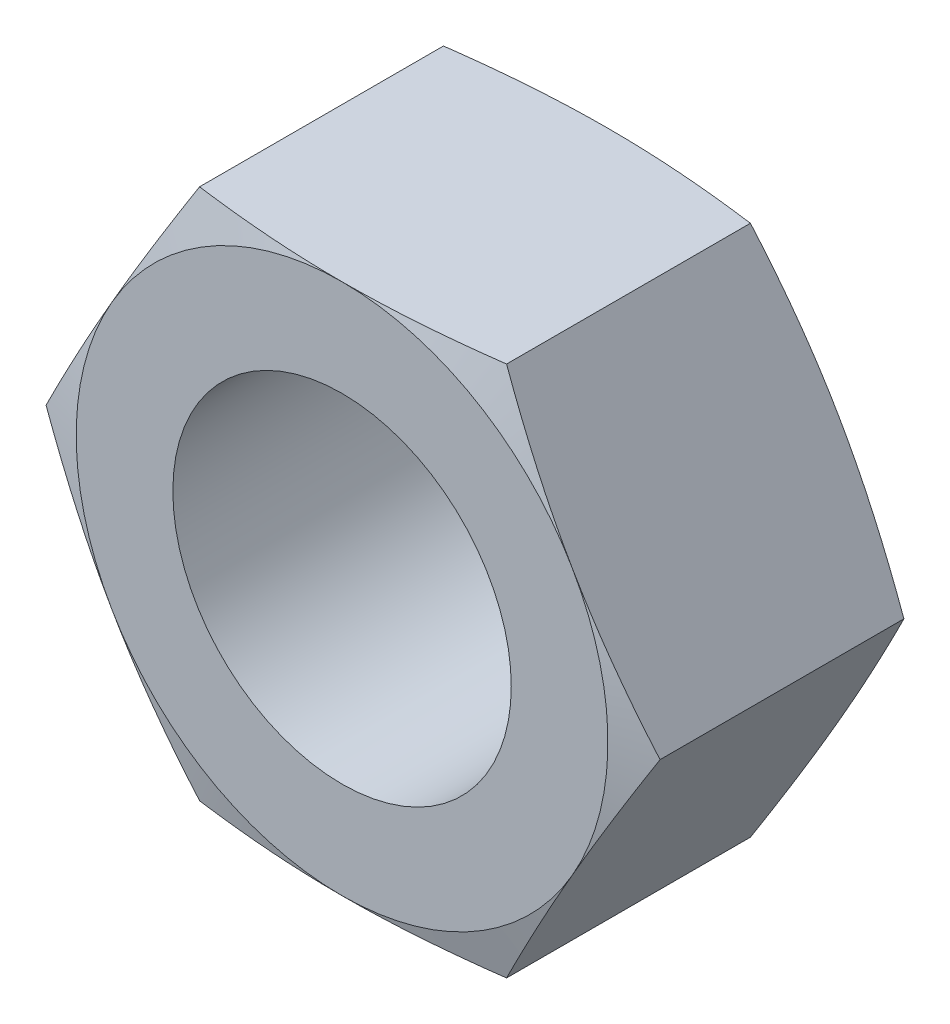
from build123d import *

# Parameters (mm, degrees)
SKETCH1_R          = 7
BASE_EXTRUDE_DEPTH = 11
SKETCH2_OUTSIDE_W  = 318.108
SKETCH2_OUTSIDE_H  = 314.706
SKETCH2_OUTSIDE_R  = 10.998522628
CUT_EXTRUDE1_DEPTH = 38
CUT_EXTRUDE1_DRAFT = -75
SKETCH3_OUTSIDE_W  = 318.108
SKETCH3_OUTSIDE_H  = 314.706
SKETCH3_OUTSIDE_R  = 10.998522628
CUT_EXTRUDE2_DEPTH = 38
CUT_EXTRUDE2_DRAFT = -75


with BuildPart() as part:
    # Sketch1 → Base-Extrude (new body)
    with BuildSketch(Plane.XY):
        Polygon((6.35, 10.998522628), (-6.35, 10.998522628), (-12.7, 0), (-6.35, -10.998522628), (6.35, -10.998522628), (12.7, 0), align=None)
        Circle(SKETCH1_R, mode=Mode.SUBTRACT)
    extrude(amount=BASE_EXTRUDE_DEPTH)


with BuildPart() as cut_extrude1_tool:
    # Sketch2 outside → Cut-Extrude1 (with draft: the straight prism first)
    with BuildSketch(Plane(origin=(0, 0, 0), x_dir=(-1, 0, 0), z_dir=(0, 0, -1))):
        Rectangle(SKETCH2_OUTSIDE_W, SKETCH2_OUTSIDE_H)
        Circle(SKETCH2_OUTSIDE_R, mode=Mode.SUBTRACT)
    extrude(amount=-CUT_EXTRUDE1_DEPTH)
    # Cut-Extrude1: the draft: its side faces are tilted about the plane it starts from
    cut_extrude1_sides = [cut_extrude1_tool.faces().sort_by_distance(p)[0] for p in [
        (0, -157.353, 19),
        (-159.054, 0, 19),
        (0, 157.353, 19),
        (159.054, 0, 19),
        (10.998522628, 0, 19),
    ]]
    draft(cut_extrude1_sides, Plane(origin=(0, 0, 0), x_dir=(-1, 0, 0), z_dir=(0, 0, -1)), CUT_EXTRUDE1_DRAFT)


with BuildPart() as part_1:
    add(part.part)

    # Cut-Extrude1: cut by cut_extrude1_tool
    add(cut_extrude1_tool.part, mode=Mode.SUBTRACT)


with BuildPart() as cut_extrude2_tool:
    # Sketch3 outside → Cut-Extrude2 (with draft: the straight prism first)
    with BuildSketch(Plane.XY.offset(11)):
        Rectangle(SKETCH3_OUTSIDE_W, SKETCH3_OUTSIDE_H)
        Circle(SKETCH3_OUTSIDE_R, mode=Mode.SUBTRACT)
    extrude(amount=-CUT_EXTRUDE2_DEPTH)
    # Cut-Extrude2: the draft: its side faces are tilted about the plane it starts from
    cut_extrude2_sides = [cut_extrude2_tool.faces().sort_by_distance(p)[0] for p in [
        (0, -157.353, -8),
        (159.054, 0, -8),
        (0, 157.353, -8),
        (-159.054, 0, -8),
        (-10.998522628, 0, -8),
    ]]
    draft(cut_extrude2_sides, Plane.XY.offset(11), CUT_EXTRUDE2_DRAFT)


with BuildPart() as part_2:
    add(part_1.part)

    # Cut-Extrude2: cut by cut_extrude2_tool
    add(cut_extrude2_tool.part, mode=Mode.SUBTRACT)


solid = part_2.part
